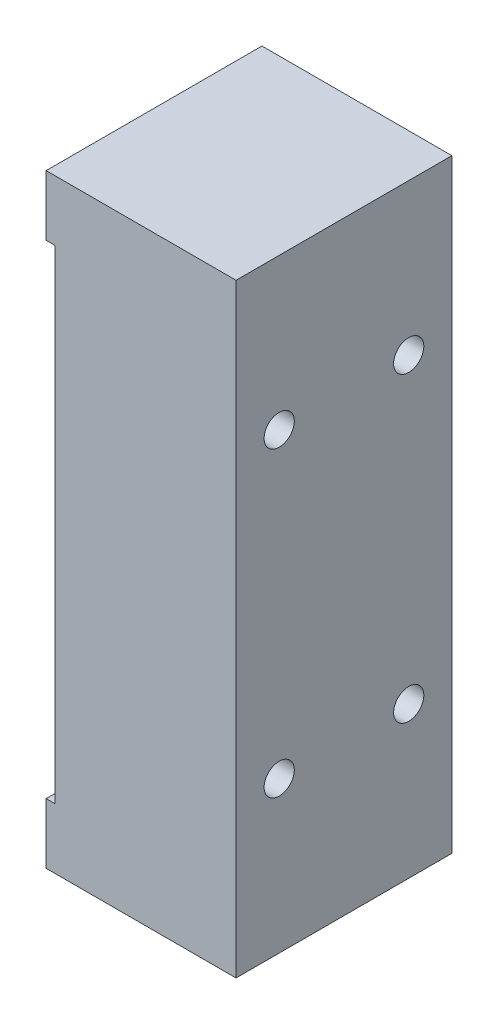
SolidWorks part; units mm, degrees
material "E-玻璃纤维"
ref_plane "Front Plane" through (0, 0, 0) normal (0, 0, 1) x (1, 0, 0)
ref_plane "Top Plane" through (0, 0, 0) normal (0, 1, 0) x (1, 0, 0)
ref_plane "Right Plane" through (0, 0, 0) normal (1, 0, 0) x (0, 0, -1)
sketch "Sketch1" plane through (0, 0, 0) normal (0, 1, 0) x (1, 0, 0)
  line L0 (0, 0) -> (0, -50000) construction
  line L1 (-11, 12.5) -> (11, 12.5)
  line L2 (-11, 12.5) -> (-11, -12.5)
  line L3 (-11, -12.5) -> (11, -12.5)
  line L4 (11, 12.5) -> (11, -12.5)
  line L5 (-11, 12.5) -> (11, -12.5) construction
  line L6 (-11, -12.5) -> (11, 12.5) construction
  line L12 (-2.45, -5) -> (2.45, -1) construction
  line L13 (-2.45, -1) -> (2.45, -5) construction
  line L18 (-2.5289, -24.1834) -> (2.05, -2.5) construction
  line L19 (-2.05, -2.5) -> (2.8719, -25.8076) construction
  point P0 (0, 0)
  point P8 (0, -3)
  point P13 (0, -12.2077)
  dimension "D1" = 22
  dimension "D2" = 25
extrude "Boss-Extrude1" add sketch "Sketch1" along normal blind 70
sketch "Sketch2" plane through (11, 0, 0) normal (1, 0, 0) x (0, 0, -1)
  line L0 (0, 0) -> (0, 50000) construction
  line L1 (-12.5, 35) -> (49987.5, 35) construction
  line L2 (-12.5, 70) -> (-12.5, 0) construction
  circle A0 centre (-7.5, 52.5) radius 1.75
  circle A1 centre (7.5, 52.5) radius 1.75
  circle A2 centre (7.5, 17.5) radius 1.75
  circle A3 centre (-7.5, 17.5) radius 1.75
  point P7 (-12.5, 35)
  dimension "D1" = 35
  dimension "D3" = 3.5
  dimension "D2" = 15
extrude "Cut-Extrude1" cut sketch "Sketch2" against normal through all
sketch "Sketch4" plane through (-11, 0, 0) normal (-1, 0, 0) x (0, 0, 1)
  line L0 (-12.5, 35) -> (49987.5, 35) construction
  line L1 (-12.5, 70) -> (-12.5, 0) construction
  line L2 (0, 60) -> (0, -49940) construction
  line L3 (-12.5, 70) -> (12.5, 70) construction
  line L4 (12.5, 70) -> (12.5, 0) construction
  line L5 (-12.5, 63) -> (12.5, 63)
  line L6 (-12.5, 63) -> (-12.5, 7)
  line L7 (-12.5, 7) -> (12.5, 7)
  line L8 (12.5, 63) -> (12.5, 7)
  line L9 (-12.5, 63) -> (12.5, 7) construction
  line L10 (-12.5, 7) -> (12.5, 63) construction
  point P4 (-12.5, 35)
  point P9 (0, 70)
  point P10 (0, 35)
  dimension "D1" = 56
extrude "Cut-Extrude3" cut sketch "Sketch4" against normal blind 1
